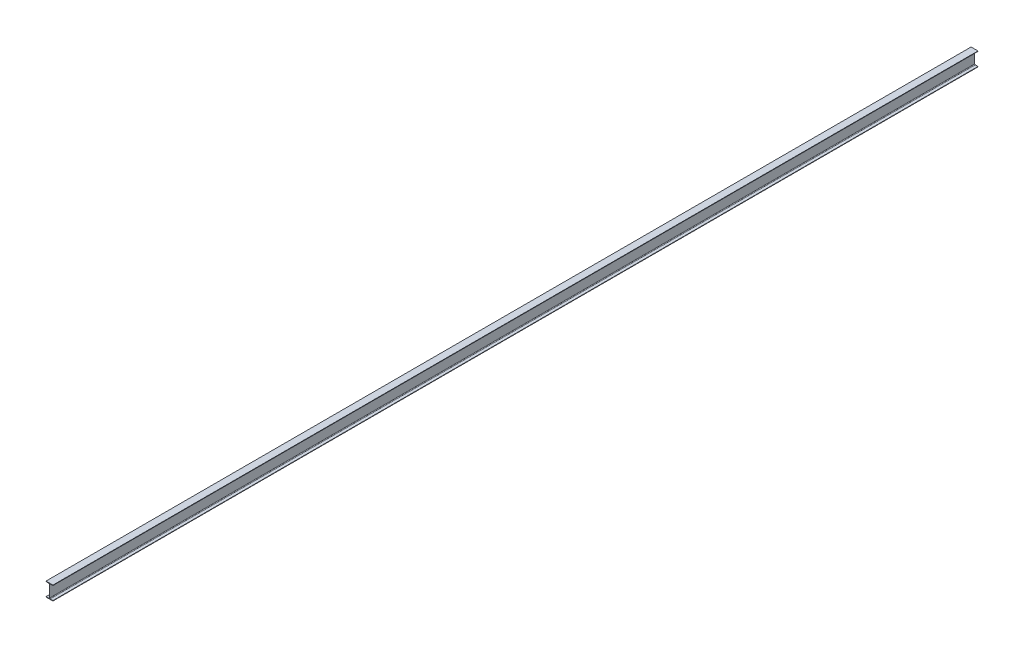
from build123d import *

# Parameters (mm, degrees)
BOSS_EXTRUDE1_DEPTH = 20067


with BuildPart() as part:
    # Sketch1 → Boss-Extrude1 (new body)
    with BuildSketch(Plane.XY):
        with BuildLine():
            Line((75, 0), (-75, 0))
            Line((-75, 0), (-75, 9))
            Line((-75, 9), (-16.25, 9))
            ThreePointArc((-16.25, 9), (-7.057611845, 12.807611845), (-3.25, 22))
            Line((-3.25, 22), (-3.25, 278))
            ThreePointArc((-3.25, 278), (-7.057611845, 287.192388155), (-16.25, 291))
            Line((-16.25, 291), (-75, 291))
            Line((-75, 291), (-75, 300))
            Line((-75, 300), (75, 300))
            Line((75, 300), (75, 291))
            Line((75, 291), (16.25, 291))
            ThreePointArc((16.25, 291), (7.057611845, 287.192388155), (3.25, 278))
            Line((3.25, 278), (3.25, 22))
            ThreePointArc((3.25, 22), (7.057611845, 12.807611845), (16.25, 9))
            Line((16.25, 9), (75, 9))
            Line((75, 9), (75, 0))
        make_face()
    extrude(amount=BOSS_EXTRUDE1_DEPTH)


solid = part.part
